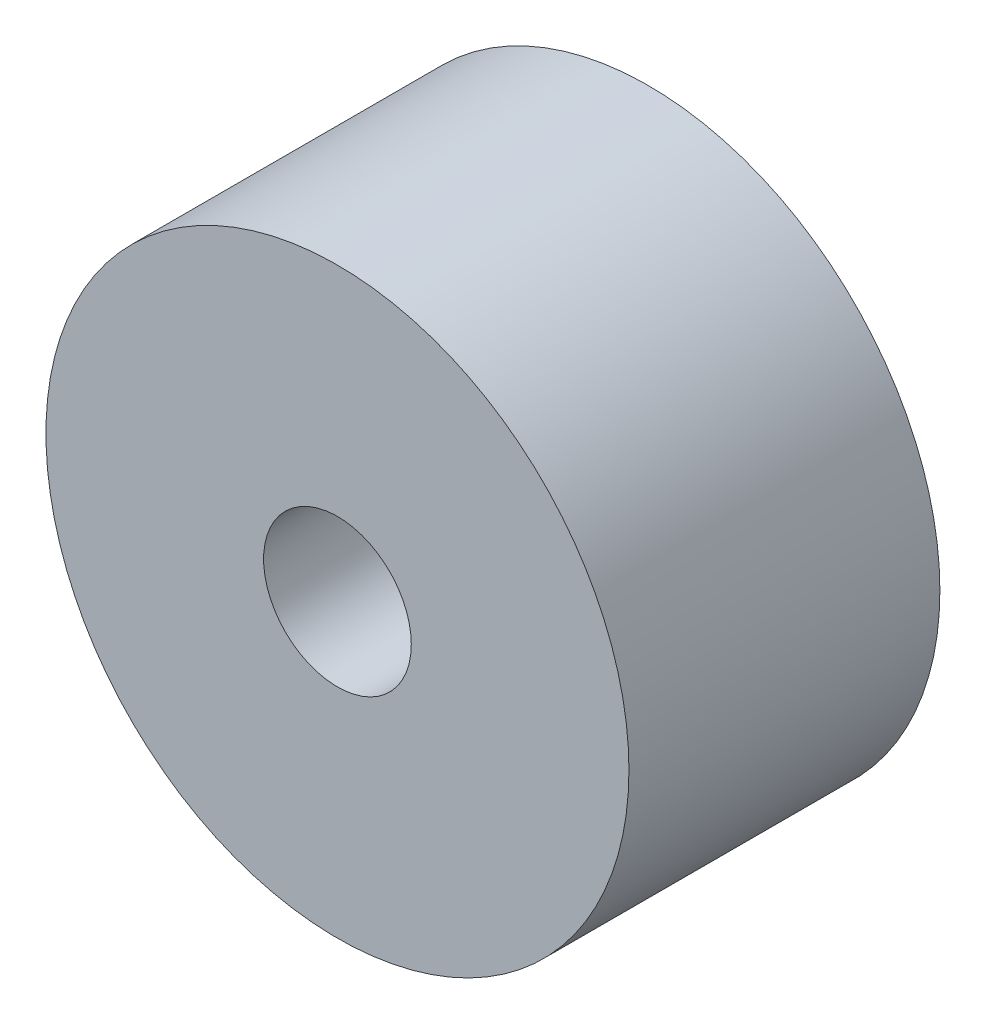
SolidWorks part; units mm, degrees
ref_plane "前视基准面" through (0, 0, 0) normal (0, 0, 1) x (1, 0, 0)
ref_plane "上视基准面" through (0, 0, 0) normal (0, 1, 0) x (1, 0, 0)
ref_plane "右视基准面" through (0, 0, 0) normal (1, 0, 0) x (0, 0, -1)
sketch "草图1" plane through (0, 0, 0) normal (0, 0, 1) x (1, 0, 0)
  circle A0 centre (0, 0) radius 38
  circle A1 centre (0, 0) radius 150
  dimension "D1" = 76
  dimension "D2" = 300
extrude "凸台-拉伸1" add sketch "草图1" along normal mid plane 160
